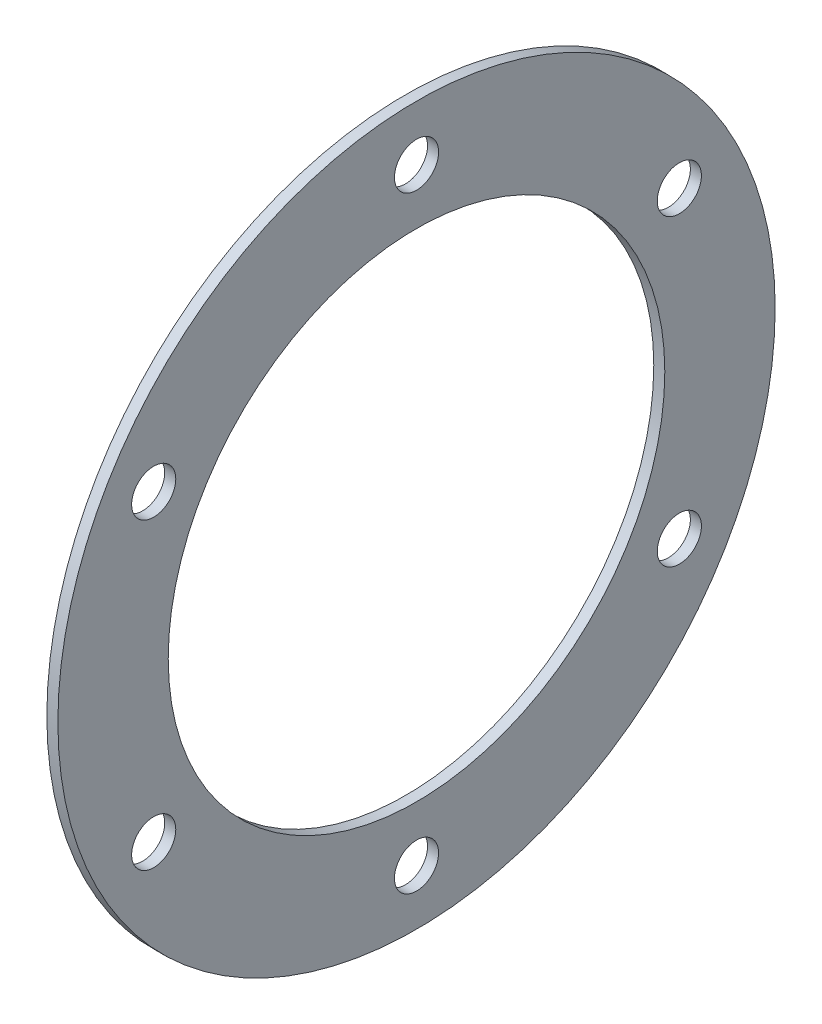
SolidWorks part; units mm, degrees
ref_plane "Front" through (0, 0, 0) normal (0, 0, 1) x (1, 0, 0)
ref_plane "Top" through (0, 0, 0) normal (0, 1, 0) x (1, 0, 0)
ref_plane "Right" through (0, 0, 0) normal (1, 0, 0) x (0, 0, -1)
sketch "Sketch1" plane through (0, 0, 0) normal (0, 0, 1) x (1, 0, 0)
  line L0 (0, 0) -> (36.4759, 0) construction
  line L1 (0, 65) -> (2, 65)
  line L2 (0, 65) -> (0, 45)
  line L3 (0, 45) -> (2, 45)
  line L4 (2, 65) -> (2, 45)
  dimension "D1" = 2
  dimension "D2" = 20
  dimension "D3" = 45
revolve "Revolve1" add sketch "Sketch1" angle 360 about L0
sketch "Sketch2" plane through (2, 0, 0) normal (1, 0, 0) x (0, 0, -1)
  line L0 (0, 0) -> (84.2407, 0) construction
  line L1 (0, 0) -> (0, 69.5202) construction
  line L2 (0, 0) -> (75.8271, 43.7788) construction
  line L3 (0, 0) -> (-73.7264, 42.5659) construction
  circle A1 centre (0, 55) radius 4
  circle A2 centre (47.6314, 27.5) radius 4
  circle A3 centre (-47.6314, 27.5) radius 4
  circle A4 centre (47.6314, -27.5) radius 4
  circle A5 centre (-47.6314, -27.5) radius 4
  circle A6 centre (0, -55) radius 4
  dimension "D4" = 8
  dimension "D5" = 8
  dimension "D6" = 8
  dimension "D1" = 60
  dimension "D2" = 60
extrude "Cut-Extrude1" cut sketch "Sketch2" against normal blind 10
scale "Scale 1" bodies to scale 102 scale about centroid uniform scaling yes scale factor 1.875
